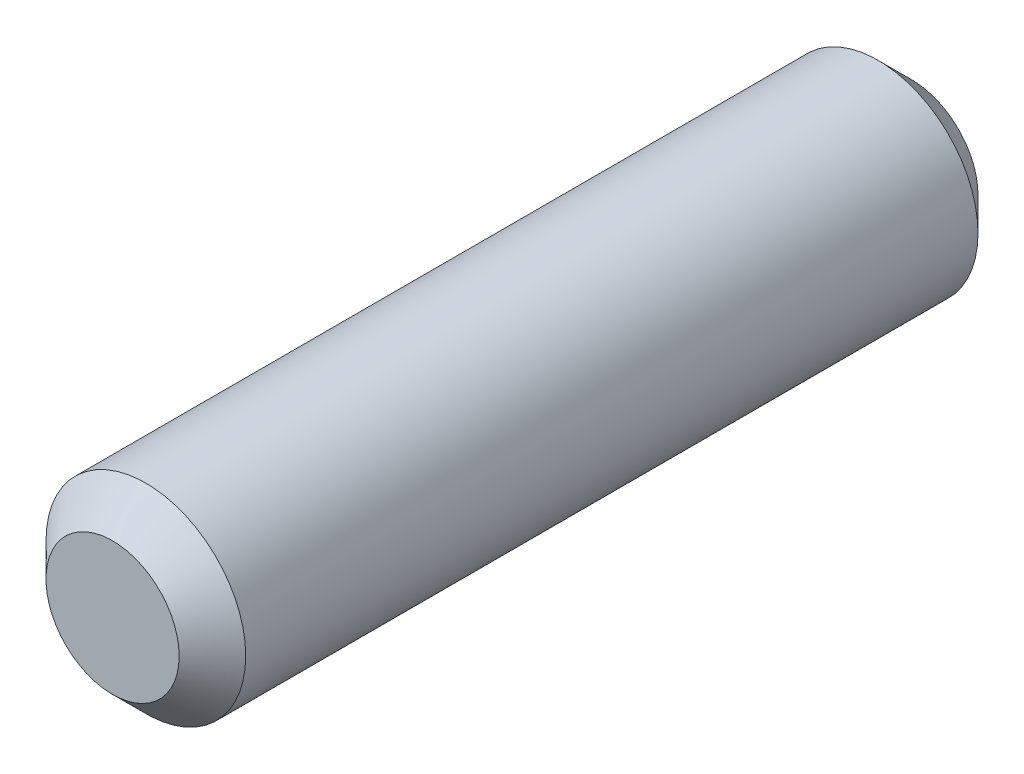
SolidWorks part; units mm, degrees
material "S45C"
ref_plane "Front Plane" through (0, 0, 0) normal (0, 0, 1) x (1, 0, 0)
ref_plane "Top Plane" through (0, 0, 0) normal (0, 1, 0) x (1, 0, 0)
ref_plane "Right Plane" through (0, 0, 0) normal (1, 0, 0) x (0, 0, -1)
sketch "Sketch1" plane through (0, 0, 0) normal (0, 0, 1) x (1, 0, 0)
  circle A0 centre (0, 0) radius 3
  dimension "D1" = 6
extrude "Boss-Extrude1" add sketch "Sketch1" along normal blind 24
chamfer "Chamfer1" distance 1 angle 45 2 edges at (3, 0, 0) (3, 0, 24)
